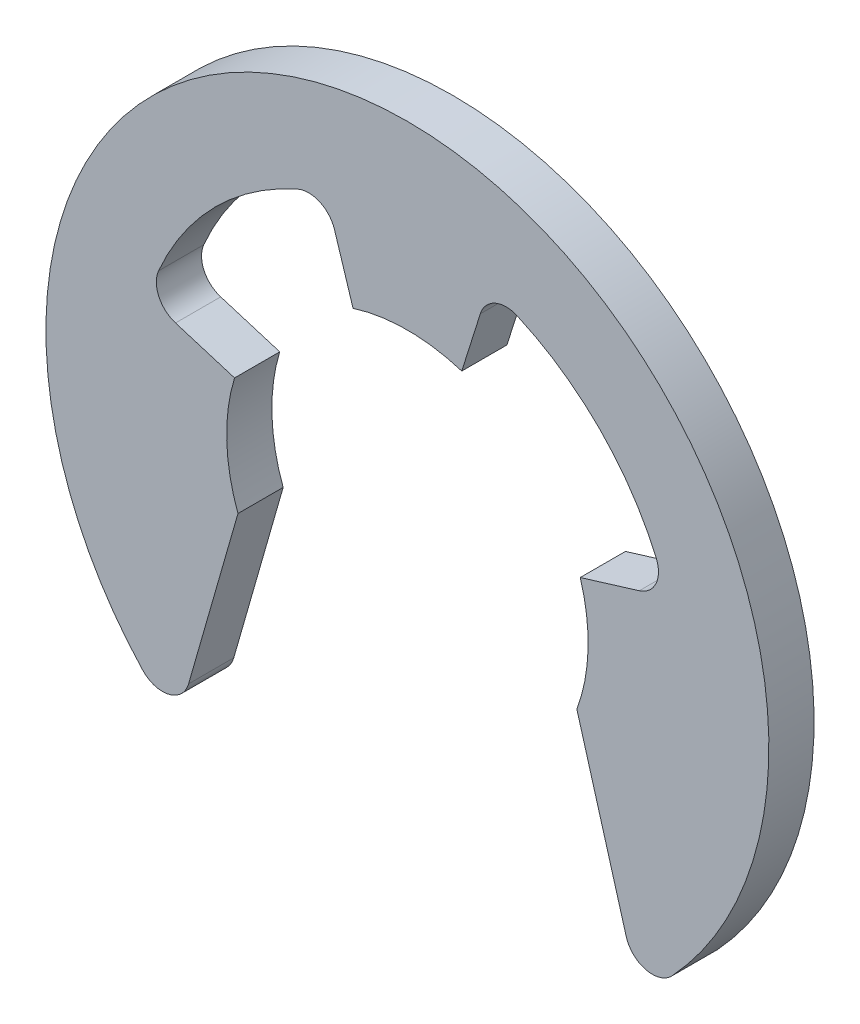
SolidWorks part; units mm, degrees
ref_plane "Front Plane" through (0, 0, 0) normal (0, 0, 1) x (1, 0, 0)
ref_plane "Top Plane" through (0, 0, 0) normal (0, 1, 0) x (1, 0, 0)
ref_plane "Right Plane" through (0, 0, 0) normal (1, 0, 0) x (0, 0, -1)
sketch "Sketch1" plane through (0, 0, 0) normal (0, 0, 1) x (1, 0, 0)
  line L0 (0, 0) -> (5.9772, 0.5229) construction
  line L1 (-2.193, 0) -> (1.9152, 0) construction
  line L2 (0, -1.8051) -> (0, 1.7867) construction
  line L3 (3.75, -1.3919) -> (4.843, -5.2038)
  line L4 (-3.75, -1.3919) -> (-4.843, -5.2038)
  line L5 (1.2028, 3.8149) -> (1.6138, 5.1182)
  line L6 (-1.2028, 3.8149) -> (-1.6138, 5.1182)
  line L7 (0, 0) -> (1.2028, 3.8149) construction
  line L8 (1.2028, 3.8149) -> (0, 0) construction
  line L9 (0, 0) -> (-1.2028, 3.8149) construction
  line L10 (3.8252, 1.1695) -> (5.1321, 1.569)
  line L11 (-3.8252, 1.1695) -> (-5.1321, 1.569)
  line L12 (0, 0) -> (3.8252, 1.1695) construction
  line L13 (3.8252, 1.1695) -> (0, 0) construction
  line L14 (0, 0) -> (-3.8252, 1.1695) construction
  arc A0 (3.75, -1.3919) -> (3.8252, 1.1695) centre (0, 0) ccw
  arc A1 (6, 0) -> (5.9772, 0.5229) centre (0, 0) ccw
  arc A2 (5.8592, -5.447) -> (-5.8592, -5.447) centre (0, 0) ccw
  arc A3 (-2.4289, 5.4864) -> (-5.5074, 2.3809) centre (0, 0) ccw
  arc A4 (-3.8252, 1.1695) -> (-3.75, -1.3919) centre (0, 0) ccw
  arc A5 (1.2028, 3.8149) -> (-1.2028, 3.8149) centre (0, 0) ccw
  arc A6 (5.5074, 2.3809) -> (2.4289, 5.4864) centre (0, 0) ccw
  arc A7 (-4.843, -5.2038) -> (-5.8592, -5.447) centre (-5.4198, -5.0384) cw
  arc A8 (5.8592, -5.447) -> (4.843, -5.2038) centre (5.4198, -5.0384) cw
  arc A9 (-5.5074, 2.3809) -> (-5.1321, 1.569) centre (-4.9566, 2.1428) ccw
  arc A10 (-1.6138, 5.1182) -> (-2.4289, 5.4864) centre (-2.186, 4.9378) ccw
  arc A11 (2.4289, 5.4864) -> (1.6138, 5.1182) centre (2.186, 4.9378) ccw
  arc A12 (5.5074, 2.3809) -> (5.1321, 1.569) centre (4.9566, 2.1428) cw
  point P22 (-5.1147, -6.1514)
  point P25 (5.1147, -6.1514)
  point P30 (-1.8042, 5.7223)
  point P33 (1.8042, 5.7223)
  point P36 (5.7378, 1.7542)
extrude "Extrude1" add sketch "Sketch1" along normal blind 1
equation "\"D4@Sketch1\" = \"D3@Sketch1\""
